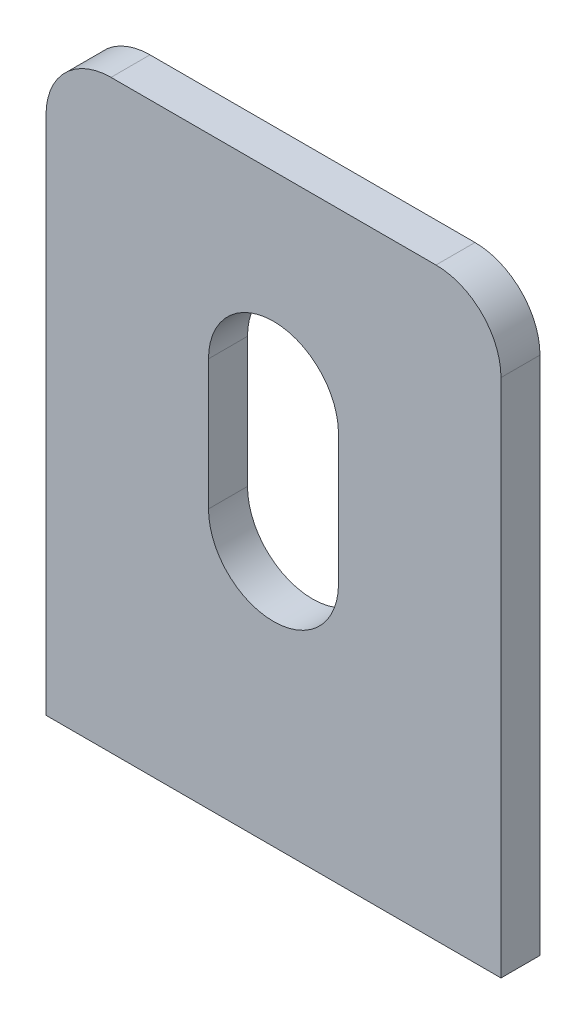
SolidWorks part; units mm, degrees
ref_plane "Front Plane" through (0, 0, 0) normal (0, 0, 1) x (1, 0, 0)
ref_plane "Top Plane" through (0, 0, 0) normal (0, 1, 0) x (1, 0, 0)
ref_plane "Right Plane" through (0, 0, 0) normal (1, 0, 0) x (0, 0, -1)
sketch "Sketch1" plane through (0, 0, 0) normal (0, 0, 1) x (1, 0, 0)
  line L0 (12.5, 30) -> (12.5, 20)
  line L1 (0, 0) -> (35, 0)
  line L2 (0, 0) -> (0, 40)
  line L3 (5, 45) -> (30, 45)
  line L4 (35, 0) -> (35, 40)
  line L5 (22.5, 30) -> (22.5, 20)
  arc A0 (12.5, 20) -> (22.5, 20) centre (17.5, 20) ccw
  arc A1 (22.5, 30) -> (12.5, 30) centre (17.5, 30) ccw
  arc A2 (0, 40) -> (5, 45) centre (5, 40) cw
  arc A3 (30, 45) -> (35, 40) centre (30, 40) cw
  point P13 (0, 45)
  dimension "D3" = 17.5
  dimension "D4" = 20
  dimension "D5" = 10
  dimension "D6" = 10
  dimension "D7" = 10
  dimension "D8" = 5
  dimension "D1" = 45
  dimension "D2" = 35
extrude "Boss-Extrude1" add sketch "Sketch1" along normal blind 3
